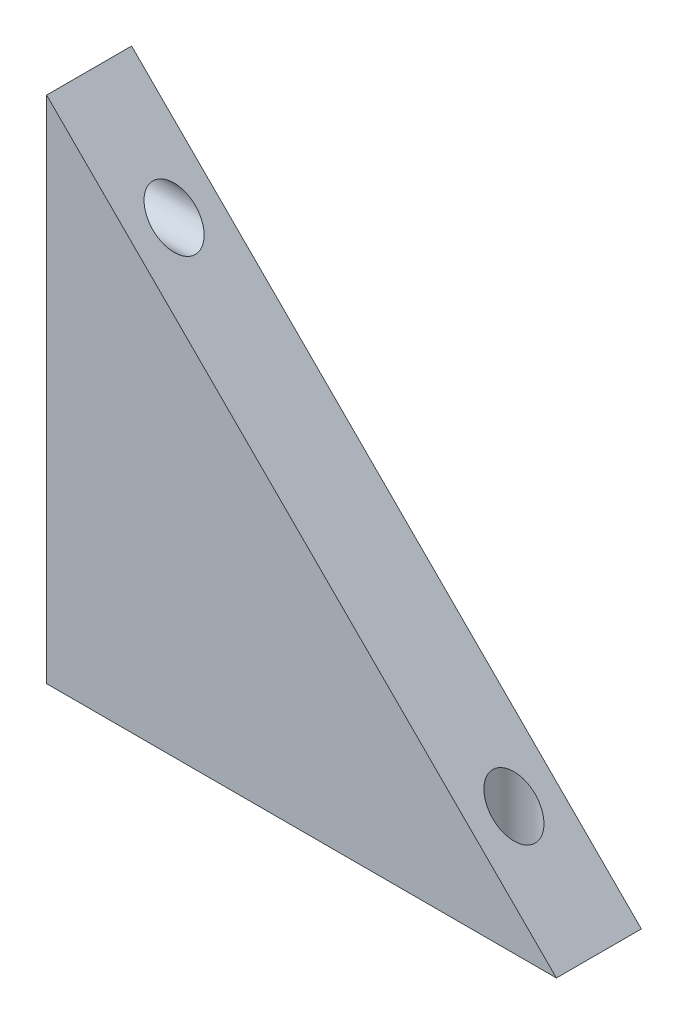
from build123d import *

# Parameters (mm, degrees)
EXTRUDE_1_DEPTH        = 10
HOLE_WIZARD_M6_2_D     = 5
HOLE_WIZARD_M6_2_DEPTH = 20
HOLE_WIZARD_M6_2_TIP   = 1.502151548
HOLE_WIZARD_M6_1_D     = 5
HOLE_WIZARD_M6_1_DEPTH = 20
HOLE_WIZARD_M6_1_TIP   = 1.502151548


with BuildPart() as part:
    # 草图1 → 凸台-拉伸1 (new body)
    with BuildSketch(Plane.XY):
        Polygon((-30, 30), (-30, -30), (30, -30), align=None)
    extrude(amount=EXTRUDE_1_DEPTH)

    # M6 螺纹孔2
    with Locations(Plane(origin=(0, -30, 0), x_dir=(-1, 0, 0), z_dir=(0, -1, 0))):
        with Locations((10, -5), (-20, -5)):
            Hole(HOLE_WIZARD_M6_2_D / 2, depth=HOLE_WIZARD_M6_2_DEPTH)
            with Locations((0, 0, -(HOLE_WIZARD_M6_2_DEPTH + HOLE_WIZARD_M6_2_TIP / 2))):  # 118° drill point
                Cone(0, HOLE_WIZARD_M6_2_D / 2, HOLE_WIZARD_M6_2_TIP, mode=Mode.SUBTRACT)

    # M6 螺纹孔1
    with Locations(Plane.ZY.offset(30)):
        with Locations((5, 20), (5, -10)):
            Hole(HOLE_WIZARD_M6_1_D / 2, depth=HOLE_WIZARD_M6_1_DEPTH)
            with Locations((0, 0, -(HOLE_WIZARD_M6_1_DEPTH + HOLE_WIZARD_M6_1_TIP / 2))):  # 118° drill point
                Cone(0, HOLE_WIZARD_M6_1_D / 2, HOLE_WIZARD_M6_1_TIP, mode=Mode.SUBTRACT)


solid = part.part
